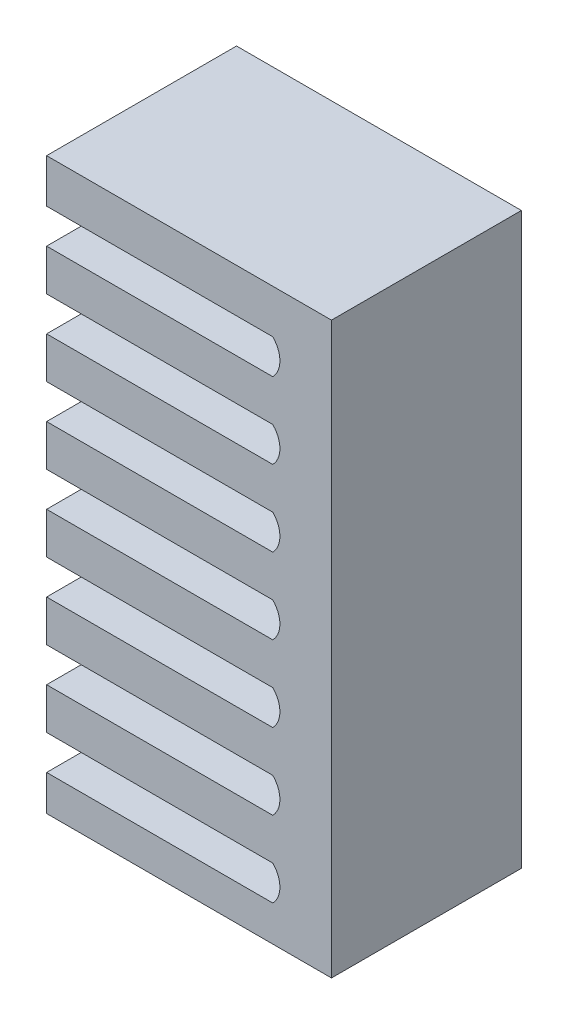
from build123d import *

# Parameters (mm, degrees)
EXTRUDE_1_DEPTH = 5


with BuildPart() as part:
    # 草图1 → 凸台-拉伸1 (new, symmetric)
    with BuildSketch(Plane.XY):
        with BuildLine():
            Line((7.5, -15), (-7.5, -15))
            Line((-7.5, -15), (-7.5, -13.125870379))
            Line((-7.5, -13.125870379), (4.407309833, -13.125870379))
            ThreePointArc((4.407309833, -13.125870379), (4.784555906, -12.215117792), (4.407309833, -11.304365204))
            Line((4.407309833, -11.304365204), (-7.5, -11.304365204))
            Line((-7.5, -11.304365204), (-7.5, -9.125870379))
            Line((-7.5, -9.125870379), (4.407309833, -9.125870379))
            ThreePointArc((4.407309833, -9.125870379), (4.784555906, -8.215117792), (4.407309833, -7.304365204))
            Line((4.407309833, -7.304365204), (-7.5, -7.304365204))
            Line((-7.5, -7.304365204), (-7.5, -5.125870379))
            Line((-7.5, -5.125870379), (4.407309833, -5.125870379))
            ThreePointArc((4.407309833, -5.125870379), (4.784555906, -4.215117792), (4.407309833, -3.304365204))
            Line((4.407309833, -3.304365204), (-7.5, -3.304365204))
            Line((-7.5, -3.304365204), (-7.5, -1.125870379))
            Line((-7.5, -1.125870379), (4.407309833, -1.125870379))
            ThreePointArc((4.407309833, -1.125870379), (4.784555906, -0.215117792), (4.407309833, 0.695634796))
            Line((4.407309833, 0.695634796), (-7.5, 0.695634796))
            Line((-7.5, 0.695634796), (-7.5, 2.874129621))
            Line((-7.5, 2.874129621), (4.407309833, 2.874129621))
            ThreePointArc((4.407309833, 2.874129621), (4.784555906, 3.784882208), (4.407309833, 4.695634796))
            Line((4.407309833, 4.695634796), (-7.5, 4.695634796))
            Line((-7.5, 4.695634796), (-7.5, 6.874129621))
            Line((-7.5, 6.874129621), (4.407309833, 6.874129621))
            ThreePointArc((4.407309833, 6.874129621), (4.784555906, 7.784882208), (4.407309833, 8.695634796))
            Line((4.407309833, 8.695634796), (-7.5, 8.695634796))
            Line((-7.5, 8.695634796), (-7.5, 10.874129621))
            Line((-7.5, 10.874129621), (4.407309833, 10.874129621))
            ThreePointArc((4.407309833, 10.874129621), (4.784555906, 11.784882208), (4.407309833, 12.695634796))
            Line((4.407309833, 12.695634796), (-7.5, 12.695634796))
            Line((-7.5, 12.695634796), (-7.5, 15))
            Line((-7.5, 15), (7.5, 15))
            Line((7.5, 15), (7.5, -15))
        make_face()
    extrude(amount=EXTRUDE_1_DEPTH, both=True)


solid = part.part
